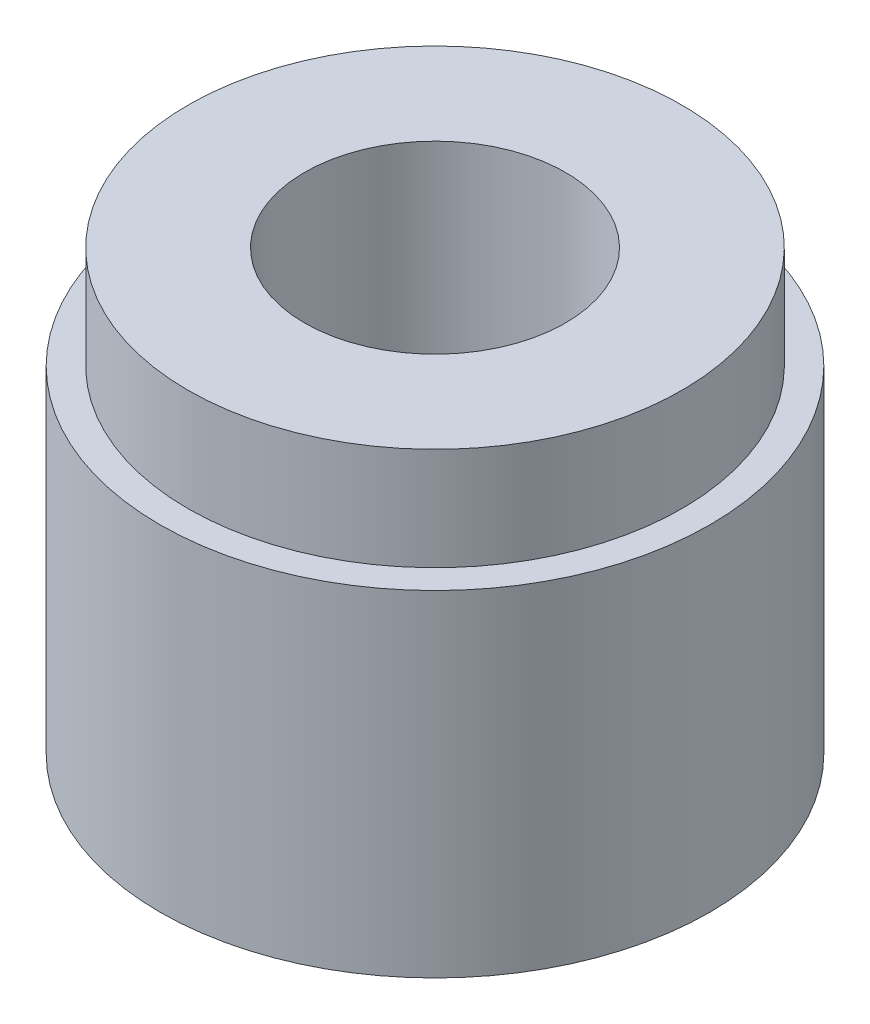
SolidWorks part; units mm, degrees
ref_plane "前视基准面" through (0, 0, 0) normal (0, 0, 1) x (1, 0, 0)
ref_plane "上视基准面" through (0, 0, 0) normal (0, 1, 0) x (1, 0, 0)
ref_plane "右视基准面" through (0, 0, 0) normal (1, 0, 0) x (0, 0, -1)
sketch "草图1" plane through (0, 0, 0) normal (0, 1, 0) x (1, 0, 0)
  circle A0 centre (0, 0) radius 59
  circle A1 centre (0, 0) radius 28
  dimension "D1" = 118
  dimension "D2" = 56
extrude "凸台-拉伸1" add sketch "草图1" along normal blind 94
sketch "草图2" plane through (0, 94, 0) normal (0, 1, 0) x (1, 0, 0)
  circle A0 centre (0, 0) radius 53
  circle A3 centre (0, 0) radius 59 construction
  dimension "D1" = 6
extrude "切除-拉伸1" cut sketch "草图2" against normal blind 22 flip side to cut
